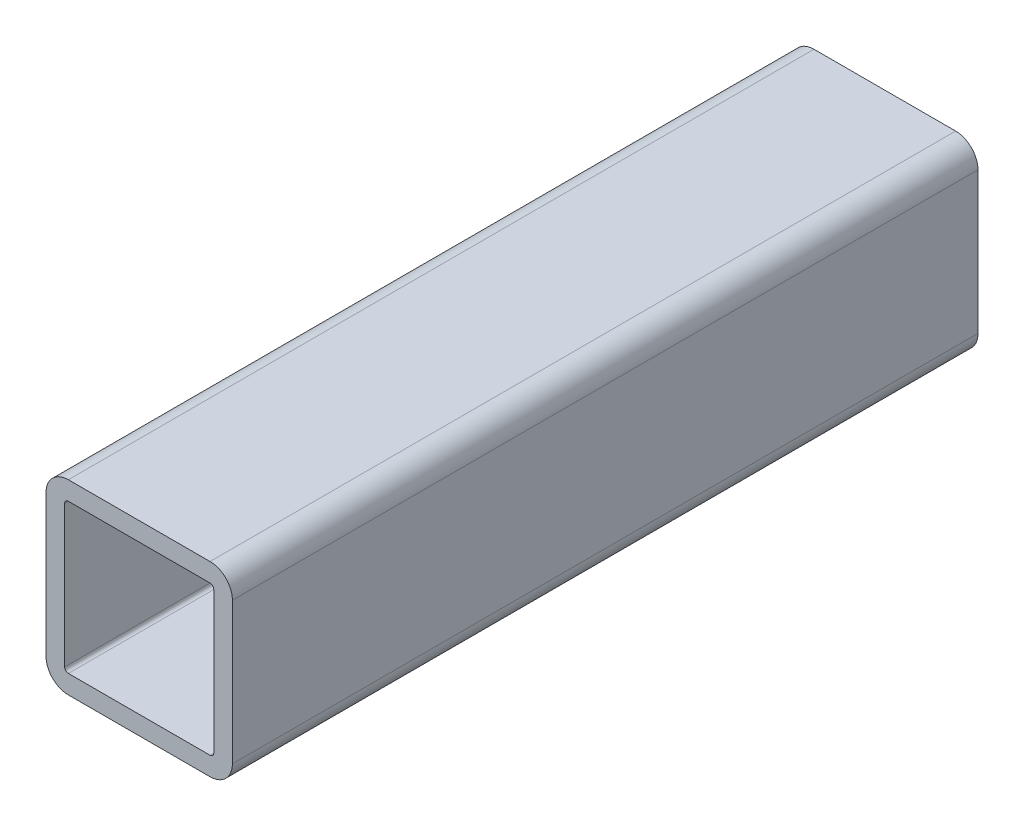
from build123d import *

# Parameters (mm, degrees)
BOSS_EXTRUDE1_DEPTH = 200


with BuildPart() as part:
    # Sketch1 → Boss-Extrude1 (new body)
    with BuildSketch(Plane.XY):
        with BuildLine():
            Line((6, 0), (44, 0))
            ThreePointArc((44, 0), (48.242640687, 1.757359313), (50, 6))
            Line((50, 6), (50, 44))
            ThreePointArc((50, 44), (48.242640687, 48.242640687), (44, 50))
            Line((44, 50), (6, 50))
            ThreePointArc((6, 50), (1.757359313, 48.242640687), (0, 44))
            Line((0, 44), (0, 6))
            ThreePointArc((0, 6), (1.757359313, 1.757359313), (6, 0))
        make_face()
        with BuildLine():
            Line((6, 45), (44, 45))
            ThreePointArc((44, 45), (44.707106781, 44.707106781), (45, 44))
            Line((45, 44), (45, 6))
            ThreePointArc((45, 6), (44.707106781, 5.292893219), (44, 5))
            Line((44, 5), (6, 5))
            ThreePointArc((6, 5), (5.292893219, 5.292893219), (5, 6))
            Line((5, 6), (5, 44))
            ThreePointArc((5, 44), (5.292893219, 44.707106781), (6, 45))
        make_face(mode=Mode.SUBTRACT)
    extrude(amount=BOSS_EXTRUDE1_DEPTH)


solid = part.part
